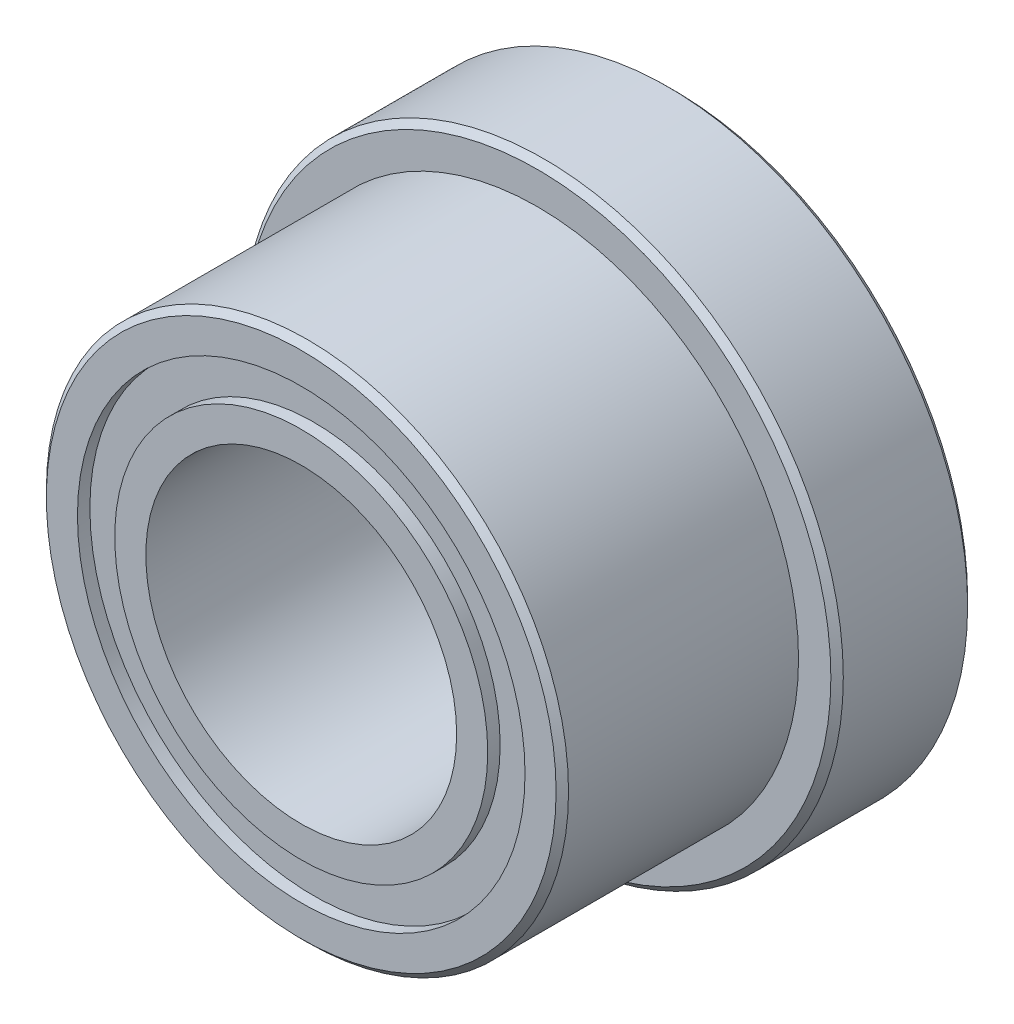
SolidWorks part; units mm, degrees
ref_plane "Front Plane" through (0, 0, 0) normal (0, 0, 1) x (1, 0, 0)
ref_plane "Top Plane" through (0, 0, 0) normal (0, 1, 0) x (1, 0, 0)
ref_plane "Right Plane" through (0, 0, 0) normal (1, 0, 0) x (0, 0, -1)
sketch "Sketch1" plane through (0, 0, 0) normal (0, 0, 1) x (1, 0, 0)
  circle A0 centre (0, 0) radius 24.1
  dimension "D1" = 48.2
extrude "Boss-Extrude1" add sketch "Sketch1" along normal blind 11
sketch "Sketch2" plane through (0, 0, 11) normal (0, 0, 1) x (1, 0, 0)
  circle A0 centre (0, 0) radius 15
  dimension "D1" = 30
extrude "Cut-Extrude1" cut sketch "Sketch2" against normal through all
sketch "Sketch3" plane through (0, 0, 11) normal (0, 0, 1) x (1, 0, 0)
  circle A0 centre (0, 0) radius 21
  circle A1 centre (0, 0) radius 12.5
  dimension "D1" = 25
  dimension "D2" = 42
extrude "Boss-Extrude2" add sketch "Sketch3" along normal blind 19
chamfer "Chamfer1" distance 0.5 angle 45 3 edges at (21, 0, 30) (24.1, 0, 11) (24.1, 0, 0)
sketch "Sketch4" plane through (0, 0, 30) normal (0, 0, 1) x (1, 0, 0)
  circle A0 centre (0, 0) radius 15
  circle A1 centre (0, 0) radius 18
  dimension "D1" = 30
  dimension "D2" = 36
extrude "Cut-Extrude2" cut sketch "Sketch4" against normal blind 1
